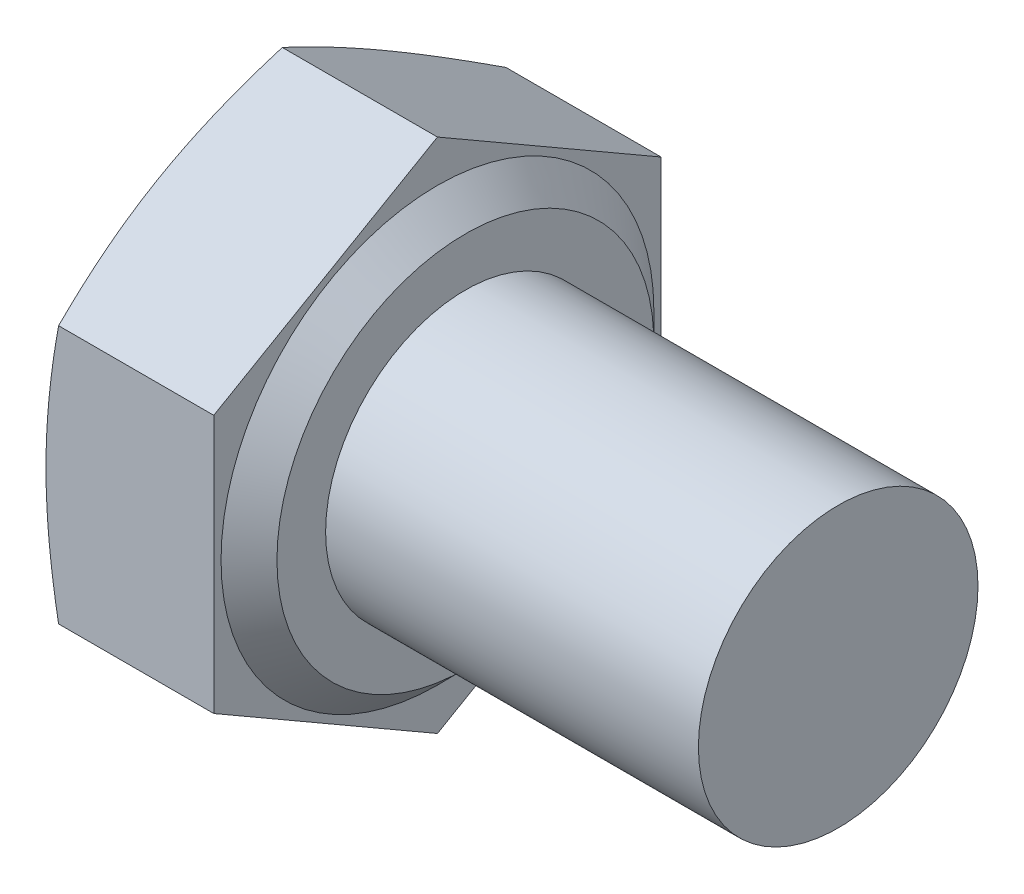
from build123d import *

# Parameters (mm, degrees)
BASEHEAD_DEPTH     = 3.5
SKETCH5_R          = 2.5
BASEBODY_DEPTH     = 10
CHAMFER1_SIZE      = 0.25
SCALE1_SCALE       = 0.6
SKETCH1_R          = 1.918221386
CUT_EXTRUDE1_DEPTH = 2


with BuildPart() as part:
    # Sketch2 → BaseHead (new body)
    with BuildSketch(Plane(origin=(0, 0, 0), x_dir=(0, 0, -1), z_dir=(1, 0, 0))):
        Polygon((0, -4.618802154), (4, -2.309401077), (4, 2.309401077), (0, 4.618802154), (-4, 2.309401077), (-4, -2.309401077), align=None)
    extrude(amount=BASEHEAD_DEPTH)

    # Sketch3 → BearingFace (revolve, cut)
    with BuildSketch(Plane.XY, mode=Mode.PRIVATE) as bearingface_sk:
        Polygon((3.5, 4.618802154), (3.5, 3.37), (3, 3.87), (3, 4.618802154), align=None)
    revolve(bearingface_sk.sketch.rotate(Axis((-0.957090588, 0, 0), (1, 0, 0)), 90), axis=Axis((-0.957090588, 0, 0), (1, 0, 0)), mode=Mode.SUBTRACT)

    # Sketch4 → HeadChamfer (revolve, cut)
    with BuildSketch(Plane.XY):
        Polygon((0, 4.618802154), (0.225225565, 4.618802154), (0, 4), align=None)
    revolve(axis=Axis((-0.493528746, 0, 0), (1, 0, 0)), mode=Mode.SUBTRACT)

    # Sketch5 → BaseBody (add)
    with BuildSketch(Plane(origin=(3.5, 0, 0), x_dir=(0, 0, -1), z_dir=(1, 0, 0))):
        with Locations(Location((0, 0, 0), (0, 0, 180))):
            Circle(SKETCH5_R)
    extrude(amount=BASEBODY_DEPTH)

    # Chamfer1
    chamfer1_edges = [part.edges().sort_by_distance(p)[0] for p in [
        (13.5, 0, -2.5),
    ]]
    chamfer(chamfer1_edges, length=CHAMFER1_SIZE)


with BuildPart() as part_1:
    # Scale1: scaled about (5.174356306, 0, 0)
    add(part.part.scale(SCALE1_SCALE).moved(Location((2.069742522, 0, 0))))

    # Sketch1 → Cut-Extrude1 (cut)
    with BuildSketch(Plane(origin=(10.169743001, 0, 0), x_dir=(0, 0, -1), z_dir=(1, 0, 0))):
        Circle(SKETCH1_R)
    extrude(amount=-CUT_EXTRUDE1_DEPTH, mode=Mode.SUBTRACT)


solid = part_1.part
